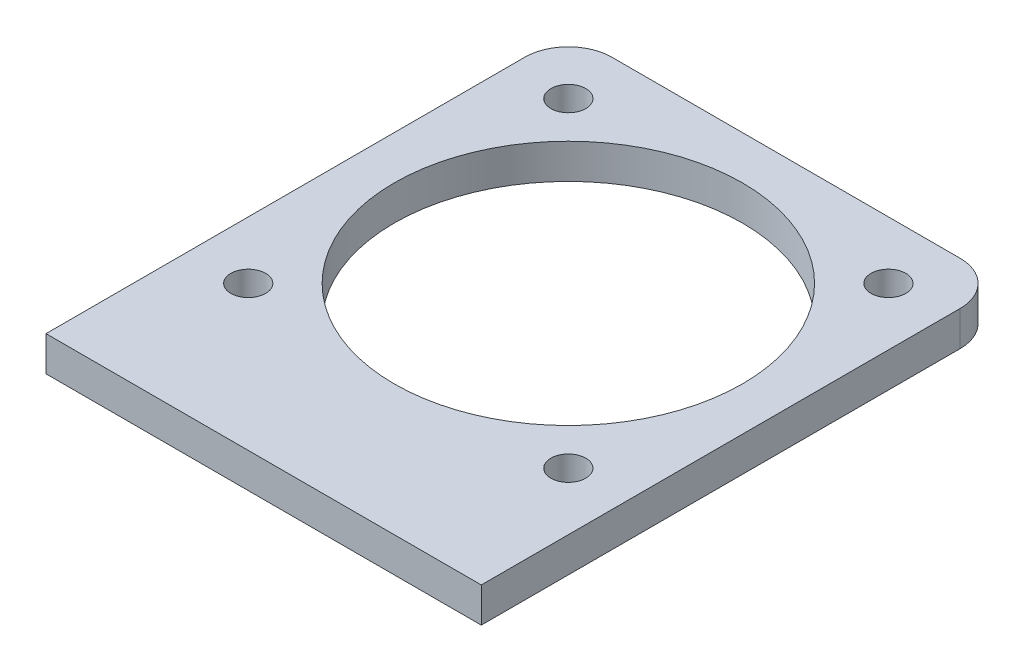
from build123d import *

# Parameters (mm, degrees)
SKETCH1_W                = 100
SKETCH1_H                = 120
BOSS_EXTRUDE1_DEPTH      = 8
FILLET1_R                = 10
CUT_EXTRUDE1_REACH       = 80.511
SKETCH2_R                = 40
F_8_0_8_DIAMETER_HOLE1_D = 8
CIRPATTERN1_COUNT        = 4


with BuildPart() as part:
    # Sketch1 → Boss-Extrude1 (new body)
    with BuildSketch(Plane(origin=(0, 0, 0), x_dir=(1, 0, 0), z_dir=(0, 1, 0))):
        Rectangle(SKETCH1_W, SKETCH1_H)
    extrude(amount=BOSS_EXTRUDE1_DEPTH)

    # Fillet1
    fillet1_edges = [part.edges().sort_by_distance(p)[0] for p in [
        (-50, 4, -60),
        (50, 4, -60),
    ]]
    fillet(fillet1_edges, radius=FILLET1_R)

    # Sketch2 → Cut-Extrude1 (cut, up to next)
    with BuildSketch(Plane(origin=(0, 8, 0), x_dir=(1, 0, 0), z_dir=(0, 1, 0)), mode=Mode.PRIVATE) as cut_extrude1_sk1:
        with Locations(Location((0, 10, 0), (0, 0, 270))):
            Circle(SKETCH2_R)
    cut_extrude1_tool1 = extrude(cut_extrude1_sk1.sketch, amount=-CUT_EXTRUDE1_REACH, mode=Mode.PRIVATE) & part.part
    add(cut_extrude1_tool1.solids().sort_by_distance((0, 8, -10))[0], mode=Mode.SUBTRACT)

    # Ø8.0 (8) Diameter Hole1 (through all)
    with Locations(Plane(origin=(0, 8, 0), x_dir=(1, 0, 0), z_dir=(0, 1, 0))):
        with Locations((-36.769552622, 46.769552622)):
            f_8_0_8_diameter_hole1 = Hole(F_8_0_8_DIAMETER_HOLE1_D / 2)

    # CirPattern1: Ø8.0 (8) Diameter Hole1 ×4 about axis
    cirpattern1_axis = Axis((0, 0, -10), (0, 1, 0))
    for i in range(1, CIRPATTERN1_COUNT):
        add(f_8_0_8_diameter_hole1.rotate(cirpattern1_axis, i * 360 / CIRPATTERN1_COUNT), mode=Mode.SUBTRACT)


solid = part.part
